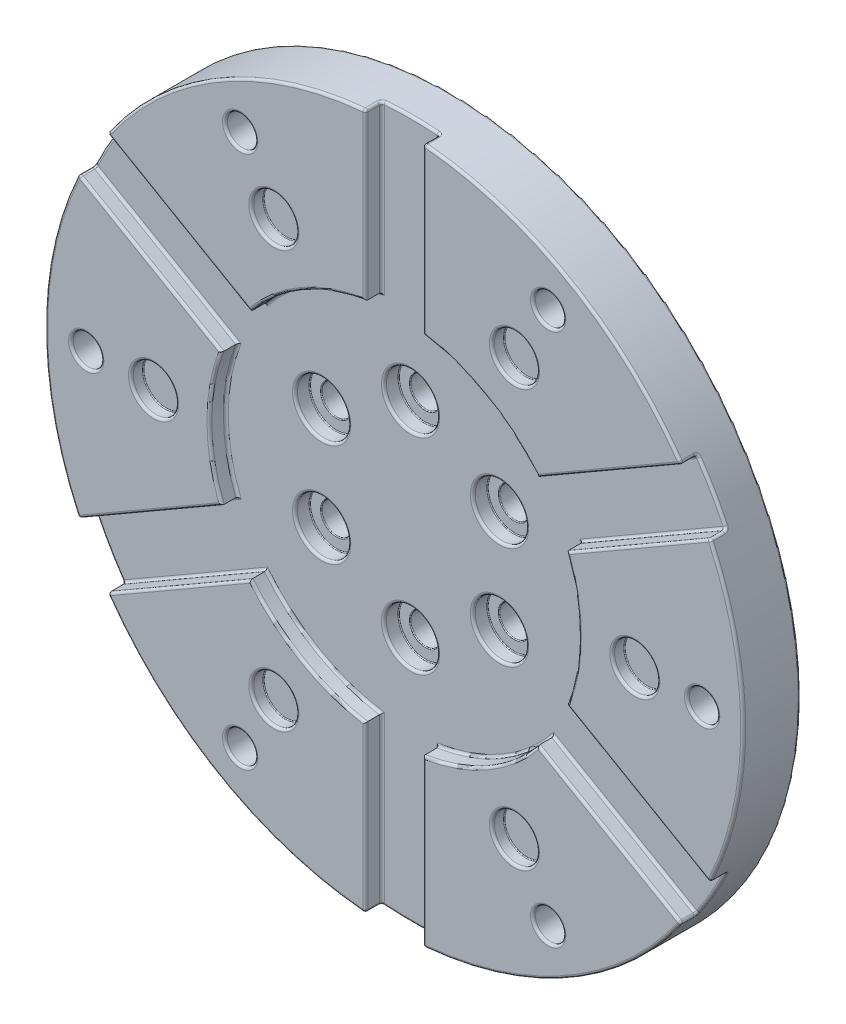
SolidWorks part; units mm, degrees
ref_plane "Front Plane" through (0, 0, 0) normal (0, 0, 1) x (1, 0, 0)
ref_plane "Top Plane" through (0, 0, 0) normal (0, 1, 0) x (1, 0, 0)
ref_plane "Right Plane" through (0, 0, 0) normal (1, 0, 0) x (0, 0, -1)
sketch "Sketch1" plane through (0, 0, 0) normal (0, 0, 1) x (1, 0, 0)
  circle A0 centre (0, 0) radius 42.5
  dimension "D1" = 85
extrude "Boss-Extrude1" add sketch "Sketch1" along normal blind 7
sketch "Sketch2" plane through (0, 0, 0) normal (0, 0, -1) x (-1, 0, 0)
  circle A0 centre (0, 0) radius 16.4
  dimension "D1" = 32.8
extrude "Boss-Extrude2" add sketch "Sketch2" along normal blind 5.3
sketch "Sketch3" plane through (0, 0, -5.3) normal (0, 0, -1) x (-1, 0, 0)
  circle A0 centre (0, 0) radius 12.5 construction
  circle A1 centre (0, 12.5) radius 1.85
  circle A2 centre (10.8253, 6.25) radius 1.85
  circle A3 centre (10.8253, -6.25) radius 1.85
  circle A4 centre (0, -12.5) radius 1.85
  circle A5 centre (-10.8253, -6.25) radius 1.85
  circle A6 centre (-10.8253, 6.25) radius 1.85
  dimension "D1" = 25
  dimension "D2" = 3.7
  dimension "D3" = 6
extrude "Cut-Extrude4" cut sketch "Sketch3" against normal through all
sketch "Sketch4" plane through (0, 0, 7) normal (0, 0, 1) x (1, 0, 0)
  circle A0 centre (0, 0) radius 37.5 construction
  circle A1 centre (-37.5, 0) radius 1.85
  circle A2 centre (-18.75, 32.476) radius 1.85
  circle A3 centre (18.75, 32.476) radius 1.85
  circle A4 centre (37.5, 0) radius 1.85
  circle A5 centre (18.75, -32.476) radius 1.85
  circle A6 centre (-18.75, -32.476) radius 1.85
  point P17 (0, 0)
  dimension "D1" = 75
  dimension "D2" = 3.7
  dimension "D3" = 6
extrude "Cut-Extrude8" cut sketch "Sketch4" against normal up to next
sketch "Sketch6" plane through (0, 0, 7) normal (0, 0, 1) x (1, 0, 0)
  line L0 (0, 0) -> (0, 44.4706) construction
  line L1 (-3.5, 44.4706) -> (3.5, 44.4706)
  line L2 (-3.5, 44.4706) -> (-3.5, 22.2261)
  line L3 (3.5, 44.4706) -> (3.5, 22.2261)
  line L4 (36.7626, 25.2664) -> (17.4984, 14.1441)
  line L5 (36.7626, 25.2664) -> (40.2626, 19.2042)
  line L6 (40.2626, 19.2042) -> (20.9984, 8.082)
  line L7 (40.2626, -19.2042) -> (20.9984, -8.082)
  line L8 (40.2626, -19.2042) -> (36.7626, -25.2664)
  line L9 (36.7626, -25.2664) -> (17.4984, -14.1441)
  line L10 (3.5, -44.4706) -> (3.5, -22.2261)
  line L11 (3.5, -44.4706) -> (-3.5, -44.4706)
  line L12 (-3.5, -44.4706) -> (-3.5, -22.2261)
  line L13 (-36.7626, -25.2664) -> (-17.4984, -14.1441)
  line L14 (-36.7626, -25.2664) -> (-40.2626, -19.2042)
  line L15 (-40.2626, -19.2042) -> (-20.9984, -8.082)
  line L16 (-40.2626, 19.2042) -> (-20.9984, 8.082)
  line L17 (-40.2626, 19.2042) -> (-36.7626, 25.2664)
  line L18 (-36.7626, 25.2664) -> (-17.4984, 14.1441)
  arc A0 (-3.5, 22.2261) -> (-17.4984, 14.1441) centre (0, 0) ccw
  arc A1 (-20.9984, 8.082) -> (-20.9984, -8.082) centre (0, 0) ccw
  arc A2 (-17.4984, -14.1441) -> (-3.5, -22.2261) centre (0, 0) ccw
  arc A3 (3.5, -22.2261) -> (17.4984, -14.1441) centre (0, 0) ccw
  arc A4 (20.9984, -8.082) -> (20.9984, 8.082) centre (0, 0) ccw
  arc A5 (17.4984, 14.1441) -> (3.5, 22.2261) centre (0, 0) ccw
  point P8 (0, 44.4706)
  point P31 (0, 0)
  dimension "D1" = 45
  dimension "D2" = 7
  dimension "D3" = 6
extrude "Cut-Extrude9" cut sketch "Sketch6" against normal blind 2
sketch "Sketch7" plane through (0, 0, 5) normal (0, 0, 1) x (1, 0, 0)
  circle A0 centre (0, 12.5) radius 3.25
  circle A1 centre (10.8253, 6.25) radius 3.25
  circle A2 centre (10.8253, -6.25) radius 3.25
  circle A3 centre (0, -12.5) radius 3.25
  circle A4 centre (-10.8253, -6.25) radius 3.25
  circle A5 centre (-10.8253, 6.25) radius 3.25
  point P15 (0, 0)
  dimension "D1" = 6.5
  dimension "D2" = 6
extrude "Cut-Extrude10" cut sketch "Sketch7" against normal blind 1.8
sketch "Sketch8" plane through (0, 0, 7) normal (0, 0, 1) x (1, 0, 0)
  line L0 (-18.75, 32.476) -> (0, 0) construction
  circle A0 centre (-14.65, 25.3745) radius 2.75
  circle A1 centre (14.65, 25.3745) radius 2.75
  circle A2 centre (29.3, 0) radius 2.75
  circle A3 centre (14.65, -25.3745) radius 2.75
  circle A4 centre (-14.65, -25.3745) radius 2.75
  circle A5 centre (-29.3, 0) radius 2.75
  point P18 (0, 0)
  dimension "D2" = 5.5
  dimension "D1" = 29.3
  dimension "D3" = 6
extrude "Cut-Extrude11" cut sketch "Sketch8" against normal blind 1.5
sketch "Sketch11" plane through (0, 0, 0) normal (0, 0, -1) x (-1, 0, 0)
  line L0 (18.75, 28.876) -> (21.8677, 30.676)
  line L1 (-15.6323, 30.676) -> (-15.6323, 34.276)
  line L2 (-15.6323, 34.276) -> (-18.75, 36.076)
  line L3 (-18.75, 36.076) -> (-21.8677, 34.276)
  line L4 (-21.8677, 34.276) -> (-21.8677, 30.676)
  line L5 (-21.8677, 30.676) -> (-18.75, 28.876)
  line L6 (-18.75, 28.876) -> (-15.6323, 30.676)
  line L7 (21.8677, 30.676) -> (21.8677, 34.276)
  line L8 (21.8677, 34.276) -> (18.75, 36.076)
  line L9 (18.75, 36.076) -> (15.6323, 34.276)
  line L10 (15.6323, 34.276) -> (15.6323, 30.676)
  line L11 (15.6323, 30.676) -> (18.75, 28.876)
  line L12 (34.3823, -1.8) -> (37.5, -3.6)
  line L13 (37.5, -3.6) -> (40.6177, -1.8)
  line L14 (40.6177, -1.8) -> (40.6177, 1.8)
  line L15 (40.6177, 1.8) -> (37.5, 3.6)
  line L16 (37.5, 3.6) -> (34.3823, 1.8)
  line L17 (34.3823, 1.8) -> (34.3823, -1.8)
  line L18 (15.6323, -30.676) -> (15.6323, -34.276)
  line L19 (15.6323, -34.276) -> (18.75, -36.076)
  line L20 (18.75, -36.076) -> (21.8677, -34.276)
  line L21 (21.8677, -34.276) -> (21.8677, -30.676)
  line L22 (21.8677, -30.676) -> (18.75, -28.876)
  line L23 (18.75, -28.876) -> (15.6323, -30.676)
  line L24 (-18.75, -28.876) -> (-21.8677, -30.676)
  line L25 (-21.8677, -30.676) -> (-21.8677, -34.276)
  line L26 (-21.8677, -34.276) -> (-18.75, -36.076)
  line L27 (-18.75, -36.076) -> (-15.6323, -34.276)
  line L28 (-15.6323, -34.276) -> (-15.6323, -30.676)
  line L29 (-15.6323, -30.676) -> (-18.75, -28.876)
  line L30 (-34.3823, 1.8) -> (-37.5, 3.6)
  line L31 (-37.5, 3.6) -> (-40.6177, 1.8)
  line L32 (-40.6177, 1.8) -> (-40.6177, -1.8)
  line L33 (-40.6177, -1.8) -> (-37.5, -3.6)
  line L34 (-37.5, -3.6) -> (-34.3823, -1.8)
  line L35 (-34.3823, -1.8) -> (-34.3823, 1.8)
  line L36 (0, 0) -> (-21.25, 36.8061) construction
  line L37 (-21.25, 36.8061) -> (-19.4567, 37.8415) construction
  circle A0 centre (-18.75, 32.476) radius 3.1177 construction
  circle A1 centre (0, 0) radius 42.5 construction
  point P41 (0, 0)
  dimension "D1" = 3.6
  dimension "D2" = 6
extrude "Cut-Extrude12" cut sketch "Sketch11" against normal blind 2.5
fillet "Fillet2" radius 0.3 123 edges at (38.4311, 18.1467, 6) (38.4311, -18.1467, 6) (34.9311, -24.2089, 6) (3.5, -42.3556, 6) (-3.5, -42.3556, 6) (-34.9311, -24.2089, 6) (-38.4311, -18.1467, 6) (-38.4311, 18.1467, 6) (-34.9311, 24.2089, 6) (-3.5, 42.3556, 6) (3.5, 42.3556, 6) (34.9311, 24.2089, 6) (29.7147, 13.1143, 5) (22.5, 0, 5) (29.7147, -13.1143, 5) (36.8061, -21.25, 5) (26.2147, -19.1765, 5) (11.25, -19.4856, 5) (3.5, -32.2909, 5) (0, -42.5, 5) (-3.5, -32.2909, 5) (-11.25, -19.4856, 5) (-26.2147, -19.1765, 5) (-36.8061, -21.25, 5) (-29.7147, -13.1143, 5) (-22.5, 0, 5) (-29.7147, 13.1143, 5) (-36.8061, 21.25, 5) (-26.2147, 19.1765, 5) (-11.25, 19.4856, 5) (-3.5, 32.2909, 5) (0, 42.5, 5) (3.5, 32.2909, 5) (11.25, 19.4856, 5) (26.2147, 19.1765, 5) (36.8061, 21.25, 5) (3.25, 12.5, 5) (-7.5753, 6.25, 5) (-7.5753, -6.25, 5) (3.25, -12.5, 5) (14.0753, -6.25, 5) (14.0753, 6.25, 5) (39.35, 0, 7) (42.5, 0, 7) (29.7147, -13.1143, 7) (22.5, 0, 7) (29.7147, 13.1143, 7) (32.05, 0, 7) (20.6, -32.476, 7) (21.25, -36.8061, 7) (3.5, -32.2909, 7) (11.25, -19.4856, 7) (26.2147, -19.1765, 7) (17.4, -25.3745, 7) (-16.9, -32.476, 7) (-21.25, -36.8061, 7) (-26.2147, -19.1765, 7) (-11.25, -19.4856, 7) (-3.5, -32.2909, 7) (-11.9, -25.3745, 7) (-35.65, 0, 7) (-42.5, 0, 7) (-29.7147, 13.1143, 7) (-22.5, 0, 7) (-29.7147, -13.1143, 7) (-26.55, 0, 7) (-16.9, 32.476, 7) (-21.25, 36.8061, 7) (-3.5, 32.2909, 7) (-11.25, 19.4856, 7) (-26.2147, 19.1765, 7) (-11.9, 25.3745, 7) (20.6, 32.476, 7) (21.25, 36.8061, 7) (26.2147, 19.1765, 7) (11.25, 19.4856, 7) (3.5, 32.2909, 7) (17.4, 25.3745, 7) (42.5, 0, 0) (-16.4, 0, 0) (-21.8677, 32.476, 0) (-20.3088, 35.176, 0) (-17.1912, 35.176, 0) (-15.6323, 32.476, 0) (-17.1912, 29.776, 0) (-20.3088, 29.776, 0) (17.1912, 35.176, 0) (20.3088, 35.176, 0) (21.8677, 32.476, 0) (20.3088, 29.776, 0) (17.1912, 29.776, 0) (15.6323, 32.476, 0) (-39.0588, -2.7, 0) (-40.6177, 0, 0) (-39.0588, 2.7, 0) (-35.9412, 2.7, 0) (-34.3823, 0, 0) (-35.9412, -2.7, 0) (-17.1912, -35.176, 0) (-20.3088, -35.176, 0) (-21.8677, -32.476, 0) (-20.3088, -29.776, 0) (-17.1912, -29.776, 0) (-15.6323, -32.476, 0) (21.8677, -32.476, 0) (20.3088, -35.176, 0) (17.1912, -35.176, 0) (15.6323, -32.476, 0) (17.1912, -29.776, 0) (20.3088, -29.776, 0) (39.0588, 2.7, 0) (40.6177, 0, 0) (39.0588, -2.7, 0) (35.9412, -2.7, 0) (34.3823, 0, 0) (35.9412, 2.7, 0) (-16.4, 0, -5.3) (-12.6753, 6.25, -5.3) (-12.6753, -6.25, -5.3) (-1.85, -12.5, -5.3) (8.9753, -6.25, -5.3) (8.9753, 6.25, -5.3) (-1.85, 12.5, -5.3)
fillet "Fillet3" radius 0.1 60 edges at (-26.55, 0, 5.5) (-11.9, 25.3745, 5.5) (17.4, 25.3745, 5.5) (32.05, 0, 5.5) (17.4, -25.3745, 5.5) (-11.9, -25.3745, 5.5) (12.6753, -6.25, 3.2) (14.0753, -6.25, 3.2) (1.85, -12.5, 3.2) (3.25, -12.5, 3.2) (12.6753, 6.25, 3.2) (14.0753, 6.25, 3.2) (1.85, 12.5, 3.2) (3.25, 12.5, 3.2) (-8.9753, 6.25, 3.2) (-7.5753, 6.25, 3.2) (-8.9753, -6.25, 3.2) (-7.5753, -6.25, 3.2) (-20.6, -32.476, 2.5) (-20.3088, -29.776, 2.5) (-21.8677, -32.476, 2.5) (-20.3088, -35.176, 2.5) (-17.1912, -35.176, 2.5) (-15.6323, -32.476, 2.5) (-17.1912, -29.776, 2.5) (16.9, -32.476, 2.5) (15.6323, -32.476, 2.5) (17.1912, -35.176, 2.5) (20.3088, -35.176, 2.5) (21.8677, -32.476, 2.5) (20.3088, -29.776, 2.5) (17.1912, -29.776, 2.5) (35.65, 0, 2.5) (35.9412, -2.7, 2.5) (39.0588, -2.7, 2.5) (40.6177, 0, 2.5) (39.0588, 2.7, 2.5) (35.9412, 2.7, 2.5) (34.3823, 0, 2.5) (16.9, 32.476, 2.5) (20.3088, 29.776, 2.5) (21.8677, 32.476, 2.5) (20.3088, 35.176, 2.5) (17.1912, 35.176, 2.5) (15.6323, 32.476, 2.5) (17.1912, 29.776, 2.5) (-20.6, 32.476, 2.5) (-15.6323, 32.476, 2.5) (-17.1912, 35.176, 2.5) (-20.3088, 35.176, 2.5) (-21.8677, 32.476, 2.5) (-20.3088, 29.776, 2.5) (-17.1912, 29.776, 2.5) (-39.35, 0, 2.5) (-35.9412, 2.7, 2.5) (-39.0588, 2.7, 2.5) (-40.6177, 0, 2.5) (-39.0588, -2.7, 2.5) (-35.9412, -2.7, 2.5) (-34.3823, 0, 2.5)
equation "\"0，1\"=0.3"
